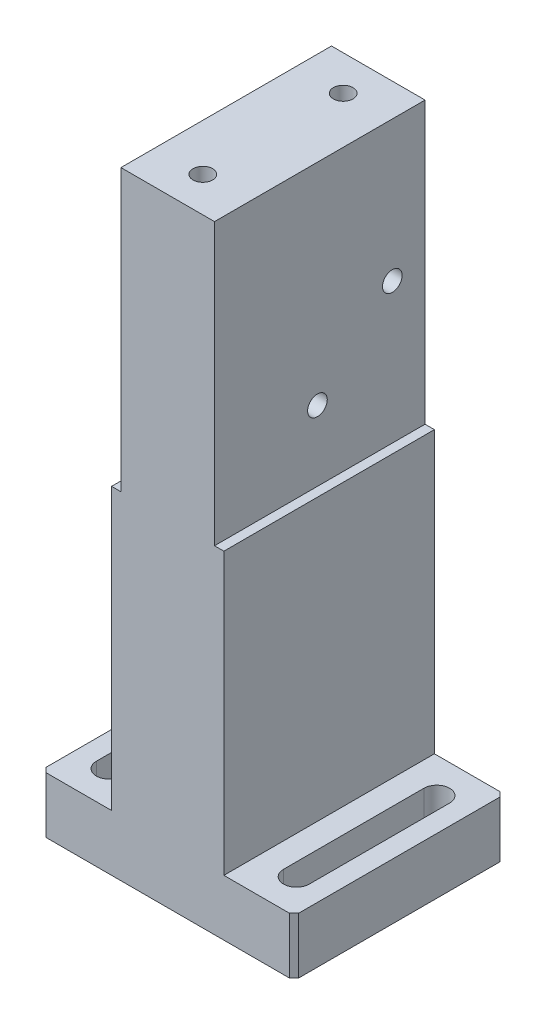
SolidWorks part; units mm, degrees
ref_plane "Front Plane" through (0, 0, 0) normal (0, 0, 1) x (1, 0, 0)
ref_plane "Top Plane" through (0, 0, 0) normal (0, 1, 0) x (1, 0, 0)
ref_plane "Right Plane" through (0, 0, 0) normal (1, 0, 0) x (0, 0, -1)
sketch "Sketch1" plane through (0, 0, 0) normal (0, 0, 1) x (1, 0, 0)
  line L0 (0, 0) -> (0, 132) construction
  line L1 (27, 0) -> (-27, 0)
  line L2 (-27, 0) -> (-27, 12)
  line L3 (-27, 12) -> (-12, 12)
  line L4 (-12, 12) -> (-12, 132)
  line L5 (-12, 132) -> (12, 132)
  line L6 (27, 0) -> (27, 12)
  line L7 (27, 12) -> (12, 12)
  line L8 (12, 12) -> (12, 132)
  dimension "D1" = 27
  dimension "D2" = 12
  dimension "D3" = 132
  dimension "D4" = 24
extrude "Boss-Extrude1" add sketch "Sketch1" along normal blind 45
sketch "Sketch9" plane through (0, 0, 45) normal (0, 0, 1) x (1, 0, 0)
  line L0 (0, 132) -> (0, 0) construction
  line L1 (-12, 132) -> (-10, 132)
  line L2 (-12, 132) -> (-12, 72)
  line L3 (-12, 72) -> (-10, 72)
  line L4 (-10, 132) -> (-10, 72)
  line L5 (12, 132) -> (-12, 132) construction
  line L6 (12, 72) -> (10, 72)
  line L7 (10, 132) -> (10, 72)
  line L8 (12, 132) -> (10, 132)
  line L9 (12, 132) -> (12, 72)
  dimension "D1" = 2
  dimension "D2" = 60
extrude "Cut-Extrude1" cut sketch "Sketch9" against normal through all
hole_wizard "M5 Tapped Hole2" positions "Sketch6" profile "Sketch5" tap size "M5" standard "Gb" end condition through all
sketch "Sketch6" plane through (10, -0.236, -1.6321) normal (1, 0, 0) x (0, 0, -1)
  line L0 (-1.6321, 72.236) -> (-46.6321, 72.236) construction
  line L1 (-1.6321, 132.236) -> (-1.6321, 72.236) construction
  point P0 (-8.6321, 102.236)
  point P1 (-24.6321, 87.236)
  dimension "D1" = 30
  dimension "D2" = 15
  dimension "D3" = 7
  dimension "D4" = 23
cosmetic thread "Cosmetic Thread4" parameters "D2"=5
cosmetic thread "Cosmetic Thread5" parameters "D2"=5
sketch "Sketch5" plane through (10, 102, 7) normal (0, 1, 0) x (0, 0, -1)
  line L0 (0, 0) -> (0, 37)
  line L1 (0, 37) -> (2.1, 37)
  line L2 (2.1, 37) -> (2.1, 0)
  line L5 (2.1, 0) -> (0, 0)
  line L11 (0, -6.35) -> (0, 107.95) construction
  dimension "通孔螺纹孔钻头直径" = 4.2
  dimension "通孔螺纹孔钻头深度" = 37
hole_wizard "Ø5.5 (5.5) Diameter Hole1" positions "Sketch8" profile "Sketch7" hole size "Ø5.5" standard "GB"
sketch "Sketch8" plane through (0, 12, 0) normal (0, 1, 0) x (-1, 0, 0)
  line L0 (0, 0) -> (0, 45) construction
  line L1 (-10, 45) -> (10, 45) construction
  line L3 (27, 22.5) -> (-27, 22.5) construction
  line L4 (27, 45) -> (27, 0) construction
  line L5 (-27, 45) -> (-27, 0) construction
  point P0 (20, 7.5)
  point P1 (20, 37.5)
  point P3 (-20, 37.5)
  point P5 (-20, 7.5)
  dimension "D1" = 40
  dimension "D2" = 30
sketch "Sketch7" plane through (-20, 12, 7.5) normal (1, 0, 0) x (0, 0, 1)
  line L0 (0, 0) -> (0, 21.6524)
  line L1 (0, 21.6524) -> (2.75, 20)
  line L2 (2.75, 20) -> (2.75, 0)
  line L5 (2.75, 0) -> (0, 0)
  line L10 (0, 21.6524) -> (-2.75, 20) construction
  line L11 (0, -6.35) -> (0, 107.95) construction
  dimension "孔直径" = 5.5
  dimension "孔深度" = 20
  dimension "导头角度" = 118
chamfer "Chamfer1" distance 1 angle 45 4 edges at (-27, 6, 45) (27, 6, 45) (27, 6, 0) (-27, 6, 0)
hole_wizard "M5 Tapped Hole3" positions "Sketch11" profile "Sketch10" tap size "M5" standard "GB"
sketch "Sketch11" plane through (0, 132, 0) normal (0, 1, 0) x (-1, 0, 0)
  line L0 (10, 22.5) -> (-10, 22.5) construction
  line L1 (10, 0) -> (10, 45) construction
  line L2 (-10, 0) -> (-10, 45) construction
  line L4 (0, 0) -> (0, 45) construction
  line L5 (-10, 45) -> (10, 45) construction
  point P0 (0, 37.5)
  point P1 (0, 7.5)
  dimension "D1" = 30
sketch "Sketch10" plane through (0, 132, 37.5) normal (1, 0, 0) x (0, 0, 1)
  line L0 (0, 0) -> (0, 15.2618)
  line L1 (0, 15.2618) -> (2.1, 14)
  line L2 (2.1, 14) -> (2.1, 0)
  line L5 (2.1, 0) -> (0, 0)
  line L10 (0, 15.2618) -> (-2.1, 14) construction
  line L11 (0, -6.35) -> (0, 107.95) construction
  dimension "螺纹孔钻头直径" = 4.2
  dimension "螺纹孔钻头深度" = 14
  dimension "导头角度" = 118
cosmetic thread "Cosmetic Thread6" parameters "D1"=10, "D2"=5
cosmetic thread "Cosmetic Thread7" parameters "D1"=10, "D2"=5
sketch "Sketch12" plane through (0, 0, 0) normal (0, -1, 0) x (1, 0, 0)
  line L0 (-20, 37.5) -> (-20, 7.5) construction
  line L1 (-17.25, 37.5) -> (-17.25, 7.5)
  line L2 (-22.75, 37.5) -> (-22.75, 7.5)
  line L3 (20, 37.5) -> (20, 7.5) construction
  line L4 (22.75, 37.5) -> (22.75, 7.5)
  line L5 (17.25, 37.5) -> (17.25, 7.5)
  arc A0 (-17.25, 37.5) -> (-22.75, 37.5) centre (-20, 37.5) ccw
  arc A1 (-22.75, 7.5) -> (-17.25, 7.5) centre (-20, 7.5) ccw
  arc A2 (22.75, 37.5) -> (17.25, 37.5) centre (20, 37.5) ccw
  arc A3 (17.25, 7.5) -> (22.75, 7.5) centre (20, 7.5) ccw
  circle A4 centre (-20, 37.5) radius 2.75 construction
  circle A5 centre (20, 37.5) radius 2.75 construction
  point P4 (-20, 22.5)
  point P13 (20, 22.5)
extrude "Cut-Extrude2" cut sketch "Sketch12" against normal up to next
